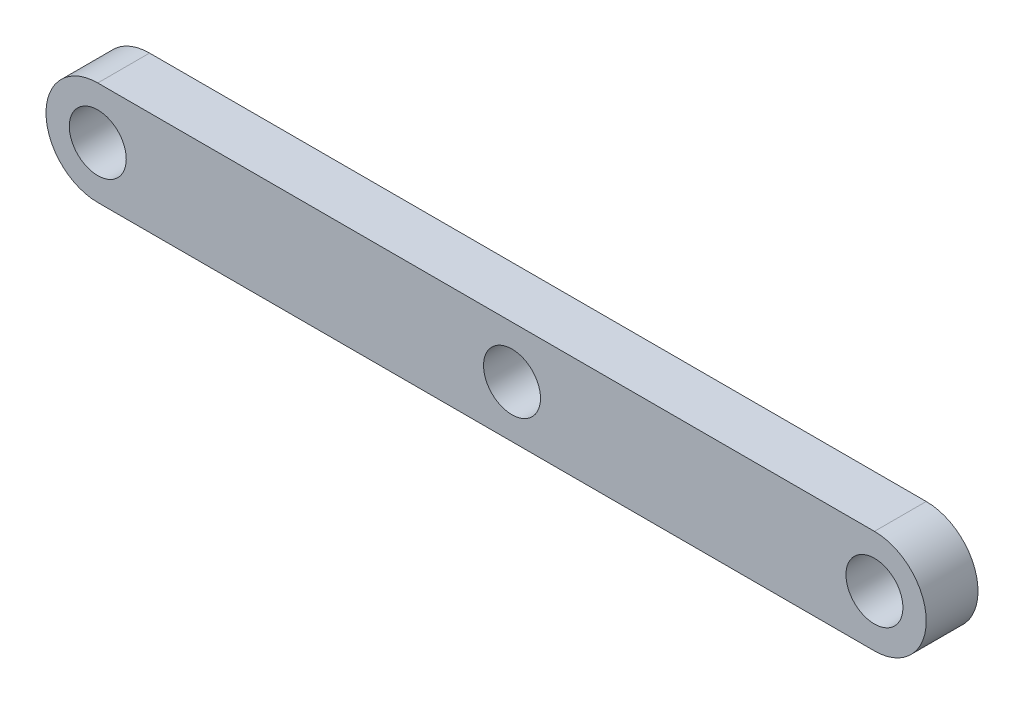
from build123d import *

# Parameters (mm, degrees)
SKETCH1_R           = 0.55
THIGH1_LENGTH_DEPTH = 0.5


with BuildPart() as part:
    # Sketch1 → Thigh1 length (new, symmetric)
    with BuildSketch(Plane.XY):
        with BuildLine():
            Line((-7.5, 1), (7.5, 1))
            ThreePointArc((7.5, 1), (8.5, 0), (7.5, -1))
            Line((7.5, -1), (-7.5, -1))
            ThreePointArc((-7.5, -1), (-8.5, 0), (-7.5, 1))
        make_face()
        with Locations((-7.5, 0)):
            Circle(SKETCH1_R, mode=Mode.SUBTRACT)
        with Locations((7.5, 0)):
            Circle(SKETCH1_R, mode=Mode.SUBTRACT)
        with Locations((0.5, 0)):
            Circle(SKETCH1_R, mode=Mode.SUBTRACT)
    extrude(amount=THIGH1_LENGTH_DEPTH, both=True)


solid = part.part
